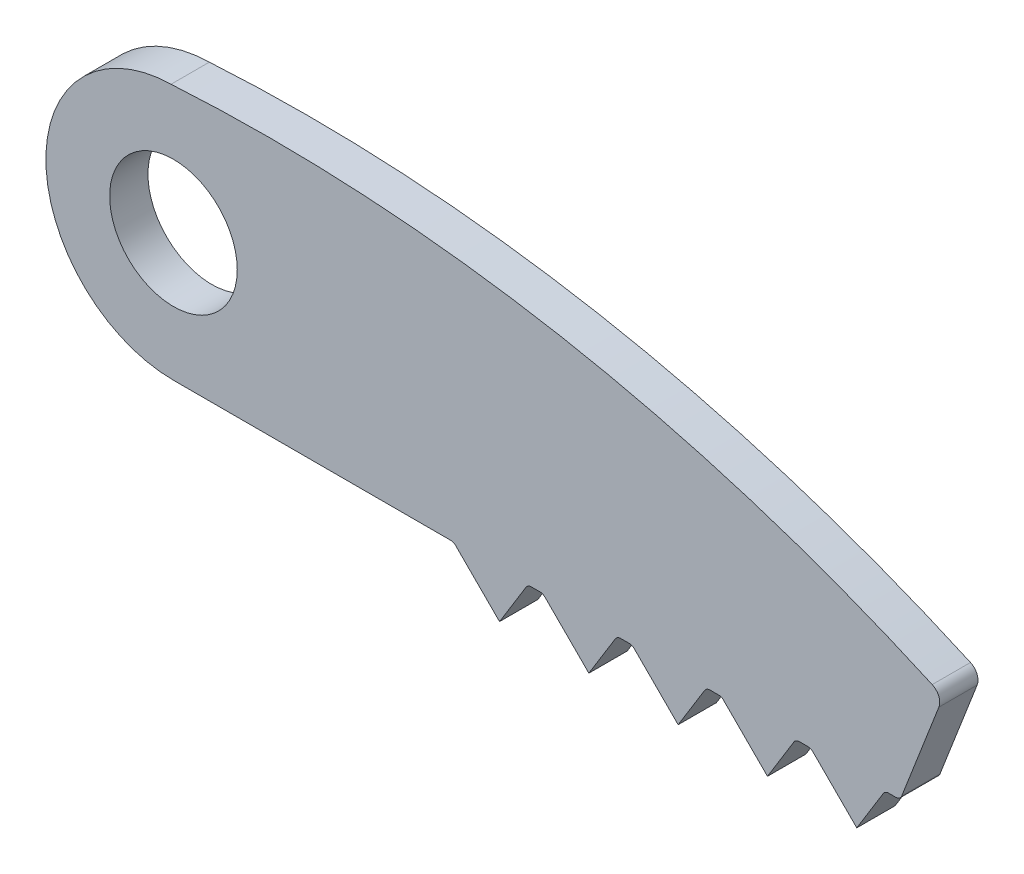
from build123d import *

# Parameters (mm, degrees)
BOSS_EXTRUDE3_DEPTH = 3
SKETCH4_R           = 5
CUT_EXTRUDE1_DEPTH  = 3


with BuildPart() as part:
    # Sketch3 → Boss-Extrude3 (new body)
    with BuildSketch(Plane.XY):
        with BuildLine():
            Line((0, -10), (21.747859728, -10))
            ThreePointArc((21.747859728, -10), (21.939201445, -10.038060234), (22.101413119, -10.146446609))
            Line((22.101413119, -10.146446609), (25.558597985, -13.603631476))
            Line((25.558597985, -13.603631476), (27.630628855, -10.237878069))
            ThreePointArc((27.630628855, -10.237878069), (27.81254922, -10.063502024), (28.056412947, -10))
            Line((28.056412947, -10), (28.747859728, -10))
            ThreePointArc((28.747859728, -10), (28.939201445, -10.038060234), (29.101413119, -10.146446609))
            Line((29.101413119, -10.146446609), (32.558597985, -13.603631476))
            Line((32.558597985, -13.603631476), (34.630628855, -10.237878069))
            ThreePointArc((34.630628855, -10.237878069), (34.81254922, -10.063502024), (35.056412947, -10))
            Line((35.056412947, -10), (35.747859728, -10))
            ThreePointArc((35.747859728, -10), (35.939201445, -10.038060234), (36.101413119, -10.146446609))
            Line((36.101413119, -10.146446609), (39.558597985, -13.603631476))
            Line((39.558597985, -13.603631476), (41.630628855, -10.237878069))
            ThreePointArc((41.630628855, -10.237878069), (41.81254922, -10.063502024), (42.056412947, -10))
            Line((42.056412947, -10), (42.747859728, -10))
            ThreePointArc((42.747859728, -10), (42.939201445, -10.038060234), (43.101413119, -10.146446609))
            Line((43.101413119, -10.146446609), (46.558597985, -13.603631476))
            Line((46.558597985, -13.603631476), (48.630628855, -10.237878069))
            ThreePointArc((48.630628855, -10.237878069), (48.81254922, -10.063502024), (49.056412947, -10))
            Line((49.056412947, -10), (49.747859728, -10))
            ThreePointArc((49.747859728, -10), (49.939201445, -10.038060234), (50.101413119, -10.146446609))
            Line((50.101413119, -10.146446609), (53.558597985, -13.603631476))
            Line((53.558597985, -13.603631476), (55.630628855, -10.237878069))
            ThreePointArc((55.630628855, -10.237878069), (55.81254922, -10.063502024), (56.056412947, -10))
            Line((56.056412947, -10), (56.612992327, -10))
            ThreePointArc((56.612992327, -10), (56.895260585, -9.912704047), (57.078965337, -9.681298521))
            Line((57.078965337, -9.681298521), (59.991284364, -2.196063373))
            ThreePointArc((59.991284364, -2.196063373), (59.984936133, -1.454957765), (59.470177564, -0.921758518))
            ThreePointArc((59.470177564, -0.921758518), (30.305424132, 8.170460374), (-0.189011515, 9.998213573))
            ThreePointArc((-0.189011515, 9.998213573), (-9.999553383, -0.094509978), (0, -10))
        make_face()
    extrude(amount=BOSS_EXTRUDE3_DEPTH)

    # Sketch4 → Cut-Extrude1 (cut)
    with BuildSketch(Plane.XY.offset(3)):
        Circle(SKETCH4_R)
    extrude(amount=-CUT_EXTRUDE1_DEPTH, mode=Mode.SUBTRACT)


solid = part.part
